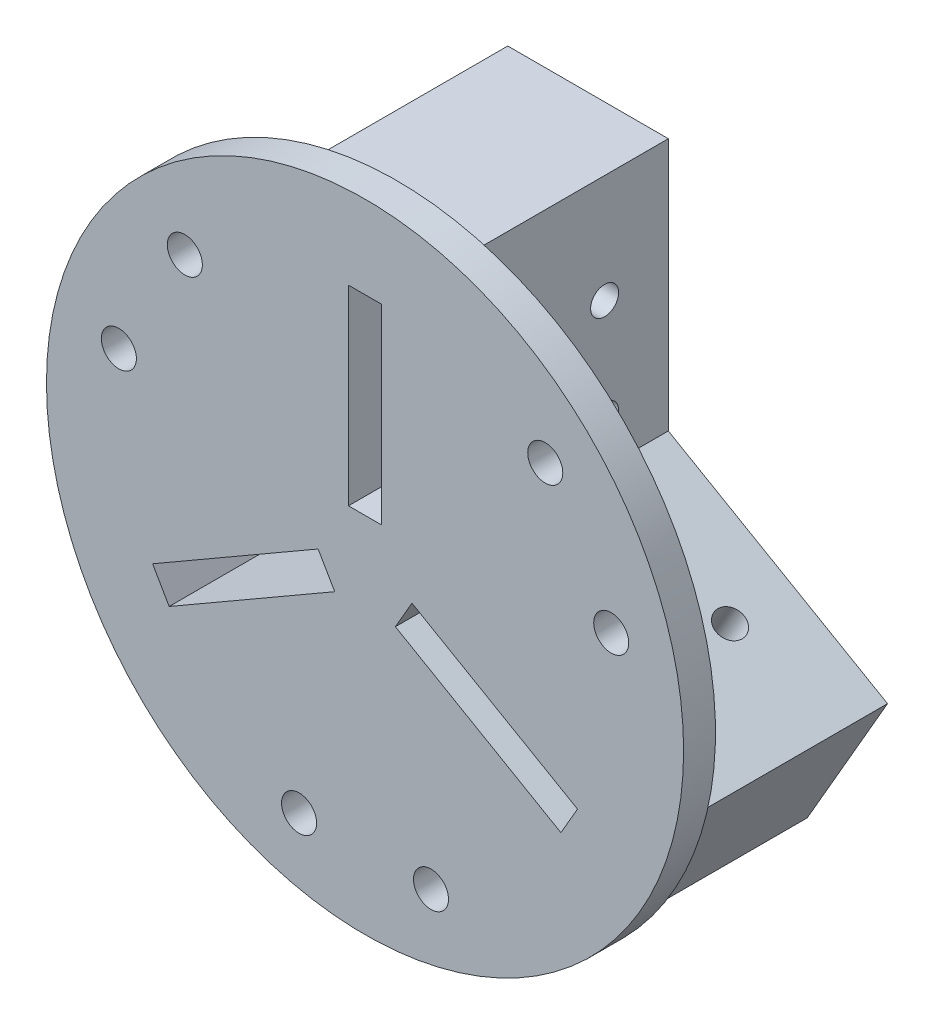
SolidWorks part; units mm, degrees
material "1.7005 (45Cr2)"
ref_plane "前视基准面" through (0, 0, 0) normal (0, 0, 1) x (1, 0, 0)
ref_plane "上视基准面" through (0, 0, 0) normal (0, 1, 0) x (1, 0, 0)
ref_plane "右视基准面" through (0, 0, 0) normal (1, 0, 0) x (0, 0, -1)
sketch "草图1" plane through (0, 0, 0) normal (0, 0, 1) x (1, 0, 0)
  line L0 (0, 22) -> (0, 0) construction
  line L1 (2.6, 7) -> (-2.6, 7)
  line L2 (2.6, 7) -> (2.6, 37)
  line L3 (2.6, 37) -> (-2.6, 37)
  line L4 (-2.6, 7) -> (-2.6, 37)
  line L5 (2.6, 7) -> (-2.6, 37) construction
  line L6 (2.6, 37) -> (-2.6, 7) construction
  line L7 (4.7622, -5.7517) -> (30.7429, -20.7517)
  line L8 (30.7429, -20.7517) -> (33.3429, -16.2483)
  line L9 (7.3622, -1.2483) -> (33.3429, -16.2483)
  line L10 (4.7622, -5.7517) -> (7.3622, -1.2483)
  line L11 (-7.3622, -1.2483) -> (-33.3429, -16.2483)
  line L12 (-33.3429, -16.2483) -> (-30.7429, -20.7517)
  line L13 (-4.7622, -5.7517) -> (-30.7429, -20.7517)
  line L14 (-7.3622, -1.2483) -> (-4.7622, -5.7517)
  circle A0 centre (0, 0) radius 50
  point P3 (0, 22)
  point P20 (0, 0)
  dimension "D1" = 100
  dimension "D2" = 30
  dimension "D3" = 5.2
  dimension "D4" = 22
  dimension "D5" = 3
extrude "凸台-拉伸1" add sketch "草图1" along normal blind 5
sketch "草图2" plane through (0, 0, 0) normal (0, 0, 1) x (1, 0, 0)
  line L4 (-2.6, 7) -> (2.6, 7)
  line L5 (-2.6, 37) -> (-2.6, 7)
  line L6 (2.6, 37) -> (-2.6, 37)
  line L7 (2.6, 7) -> (2.6, 37)
  line L8 (-2.6, 7) -> (2.6, 7)
  line L9 (-2.6, 37) -> (-2.6, 7)
  line L10 (2.6, 37) -> (-2.6, 37)
  line L11 (2.6, 7) -> (2.6, 37)
  line L12 (7.3622, -1.2483) -> (4.7622, -5.7517)
  line L13 (33.3429, -16.2483) -> (7.3622, -1.2483)
  line L14 (30.7429, -20.7517) -> (33.3429, -16.2483)
  line L15 (4.7622, -5.7517) -> (30.7429, -20.7517)
  line L16 (7.3622, -1.2483) -> (4.7622, -5.7517)
  line L17 (33.3429, -16.2483) -> (7.3622, -1.2483)
  line L18 (30.7429, -20.7517) -> (33.3429, -16.2483)
  line L19 (4.7622, -5.7517) -> (30.7429, -20.7517)
  line L20 (-4.7622, -5.7517) -> (-7.3622, -1.2483)
  line L21 (-30.7429, -20.7517) -> (-4.7622, -5.7517)
  line L22 (-33.3429, -16.2483) -> (-30.7429, -20.7517)
  line L23 (-7.3622, -1.2483) -> (-33.3429, -16.2483)
  line L24 (-4.7622, -5.7517) -> (-7.3622, -1.2483)
  line L25 (-30.7429, -20.7517) -> (-4.7622, -5.7517)
  line L26 (-33.3429, -16.2483) -> (-30.7429, -20.7517)
  line L27 (-7.3622, -1.2483) -> (-33.3429, -16.2483)
  circle A0 centre (0, 0) radius 60
  dimension "D1" = 120
  dimension "D2" = 0
  dimension "D3" = 0
  dimension "D4" = 0
extrude "凸台-拉伸2" add sketch "草图2" against normal blind 10
sketch "草图4" plane through (0, 0, -10) normal (0, 0, -1) x (-1, 0, 0)
  line L7 (-12.6, -3) -> (12.6, -3)
  line L8 (12.6, -3) -> (12.6, 47)
  line L9 (12.6, 47) -> (-12.6, 47)
  line L10 (-12.6, 47) -> (-12.6, -3)
  line L11 (-2.6, 7) -> (2.6, 7)
  line L12 (-2.6, 37) -> (-2.6, 7)
  line L13 (2.6, 37) -> (-2.6, 37)
  line L14 (2.6, 7) -> (2.6, 37)
  line L15 (-2.6, 7) -> (2.6, 7)
  line L16 (-2.6, 37) -> (-2.6, 7)
  line L17 (2.6, 37) -> (-2.6, 37)
  line L18 (2.6, 7) -> (2.6, 37)
  line L19 (-4.7622, -5.7517) -> (-7.3622, -1.2483)
  line L20 (-30.7429, -20.7517) -> (-4.7622, -5.7517)
  line L21 (-33.3429, -16.2483) -> (-30.7429, -20.7517)
  line L22 (-7.3622, -1.2483) -> (-33.3429, -16.2483)
  line L23 (-4.7622, -5.7517) -> (-7.3622, -1.2483)
  line L24 (-30.7429, -20.7517) -> (-4.7622, -5.7517)
  line L25 (-33.3429, -16.2483) -> (-30.7429, -20.7517)
  line L26 (-7.3622, -1.2483) -> (-33.3429, -16.2483)
  line L27 (7.3622, -1.2483) -> (4.7622, -5.7517)
  line L28 (33.3429, -16.2483) -> (7.3622, -1.2483)
  line L29 (30.7429, -20.7517) -> (33.3429, -16.2483)
  line L30 (4.7622, -5.7517) -> (30.7429, -20.7517)
  line L31 (7.3622, -1.2483) -> (4.7622, -5.7517)
  line L32 (33.3429, -16.2483) -> (7.3622, -1.2483)
  line L33 (30.7429, -20.7517) -> (33.3429, -16.2483)
  line L34 (4.7622, -5.7517) -> (30.7429, -20.7517)
  line L35 (8.8981, -9.4119) -> (-3.7019, 12.4119)
  line L36 (-3.7019, 12.4119) -> (-47.0032, -12.5881)
  line L37 (-47.0032, -12.5881) -> (-34.4032, -34.4119)
  line L38 (-34.4032, -34.4119) -> (8.8981, -9.4119)
  line L39 (3.7019, 12.4119) -> (-8.8981, -9.4119)
  line L40 (-8.8981, -9.4119) -> (34.4032, -34.4119)
  line L41 (34.4032, -34.4119) -> (47.0032, -12.5881)
  line L42 (47.0032, -12.5881) -> (3.7019, 12.4119)
  circle A1 centre (0, 0) radius 60
  circle M25 centre (0, 0) radius 60
  dimension "D1" = 0
  dimension "D2" = 0
  dimension "D3" = 0
  dimension "D4" = 10
extrude "切除-拉伸1" cut sketch "草图4" against normal blind 10 contours L42 L41 L40 L38 L37 L36 L10 L9 L8 M25
sketch "草图8" plane through (0, 0, -10) normal (0, 0, -1) x (-1, 0, 0)
  line L4 (-2.6, 7) -> (2.6, 7)
  line L5 (-2.6, 37) -> (-2.6, 7)
  line L6 (2.6, 37) -> (-2.6, 37)
  line L7 (2.6, 7) -> (2.6, 37)
  line L8 (-2.6, 7) -> (2.6, 7)
  line L9 (47.0032, -12.5881) -> (12.6, 7.2746)
  line L10 (12.6, 7.2746) -> (12.6, 47)
  line L11 (12.6, 47) -> (-12.6, 47)
  line L12 (-12.6, 47) -> (-12.6, 7.2746)
  line L13 (-12.6, 7.2746) -> (-47.0032, -12.5881)
  line L14 (-47.0032, -12.5881) -> (-34.4032, -34.4119)
  line L15 (-34.4032, -34.4119) -> (0, -14.5492)
  line L16 (0, -14.5492) -> (34.4032, -34.4119)
  line L17 (34.4032, -34.4119) -> (47.0032, -12.5881)
  line L18 (47.0032, -12.5881) -> (12.6, 7.2746)
  line L19 (12.6, 7.2746) -> (12.6, 47)
  line L20 (12.6, 47) -> (-12.6, 47)
  line L21 (-12.6, 47) -> (-12.6, 7.2746)
  line L22 (-12.6, 7.2746) -> (-47.0032, -12.5881)
  line L23 (-47.0032, -12.5881) -> (-34.4032, -34.4119)
  line L24 (-34.4032, -34.4119) -> (0, -14.5492)
  line L25 (0, -14.5492) -> (34.4032, -34.4119)
  line L26 (34.4032, -34.4119) -> (47.0032, -12.5881)
  line L28 (-2.6, 37) -> (-2.6, 7)
  line L29 (2.6, 37) -> (-2.6, 37)
  line L31 (2.6, 7) -> (2.6, 37)
  line L32 (-4.7622, -5.7517) -> (-7.3622, -1.2483)
  line L34 (-30.7429, -20.7517) -> (-4.7622, -5.7517)
  line L35 (-33.3429, -16.2483) -> (-30.7429, -20.7517)
  line L37 (-7.3622, -1.2483) -> (-33.3429, -16.2483)
  line L41 (-4.7622, -5.7517) -> (-7.3622, -1.2483)
  line L48 (-30.7429, -20.7517) -> (-4.7622, -5.7517)
  line L49 (-33.3429, -16.2483) -> (-30.7429, -20.7517)
  line L50 (-7.3622, -1.2483) -> (-33.3429, -16.2483)
  line L51 (7.3622, -1.2483) -> (4.7622, -5.7517)
  line L52 (33.3429, -16.2483) -> (7.3622, -1.2483)
  line L53 (30.7429, -20.7517) -> (33.3429, -16.2483)
  line L54 (4.7622, -5.7517) -> (30.7429, -20.7517)
  line L55 (7.3622, -1.2483) -> (4.7622, -5.7517)
  line L56 (33.3429, -16.2483) -> (7.3622, -1.2483)
  line L57 (30.7429, -20.7517) -> (33.3429, -16.2483)
  line L58 (4.7622, -5.7517) -> (30.7429, -20.7517)
  dimension "D1" = 0
  dimension "D2" = 0
  dimension "D3" = 0
  dimension "D4" = 0
extrude "凸台-拉伸5" add sketch "草图8" along normal blind 20
sketch "草图6" plane through (6.3, -10.9119, 0) normal (0.5, -0.866, 0) x (0.866, 0.5, 0)
  circle A4 centre (-30, -20) radius 2.2
  circle A5 centre (-14, -20) radius 2.2
extrude "切除-拉伸2" cut sketch "草图6" against normal blind 42
pattern_circular "阵列(圆周)1" count 3 over 360 about axis through (0, 0, 5) along (0, 0, -1) of "切除-拉伸2"
sketch "草图9" plane through (0, 0, 0) normal (0, 0, -1) x (-1, 0, 0)
  line L0 (0, 0) -> (28.2843, 28.2843) construction
  line L1 (0, 0) -> (38.637, 10.3528) construction
  line L2 (0, 0) -> (47.5427, 27.4488) construction
  line L4 (12.6, 7.2746) -> (12.6, 47) construction
  circle A0 centre (28.2843, 28.2843) radius 2.75
  circle A1 centre (38.637, 10.3528) radius 2.75
  dimension "D4" = 5.5
  dimension "D1" = 30
  dimension "D2" = 60
  dimension "D3" = 15
  dimension "D5" = 40
extrude "切除-拉伸3" cut sketch "草图9" against normal blind 10
sketch "草图10" plane through (0, 0, 0) normal (0, 0, -1) x (-1, 0, 0)
  circle A0 centre (28.2843, 28.2843) radius 6
  circle A1 centre (38.637, 10.3528) radius 6
  dimension "D1" = 12
extrude "切除-拉伸4" cut sketch "草图10" against normal blind 0.5
pattern_circular "阵列(圆周)2" count 3 over 360 about axis through (0, 0, 0) along (0, 0, 1) of "切除-拉伸4", "切除-拉伸3"
